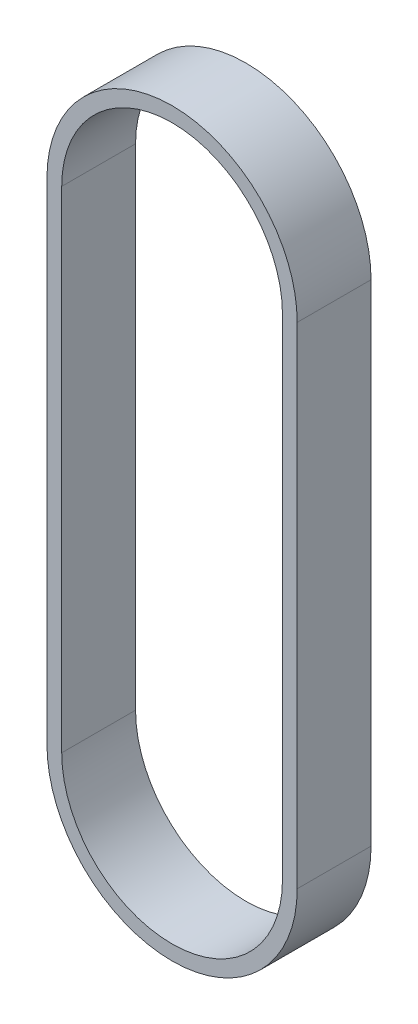
from build123d import *

# Parameters (mm, degrees)
EXTRUDE_THIN1_DEPTH = 10


with BuildPart() as part:
    # Sketch2 → Extrude-Thin1 (new body)
    with BuildSketch(Plane.XY):
        with BuildLine():
            Line((-30.341760221, -69.425568872), (-30.341760221, -3.000568872))
            ThreePointArc((-30.341760221, -3.000568872), (-13.396760221, 13.944431128), (3.548239779, -3.000568872))
            Line((3.548239779, -3.000568872), (3.548239779, -69.425568872))
            ThreePointArc((3.548239779, -69.425568872), (-13.396760221, -86.370568872), (-30.341760221, -69.425568872))
        make_face()
        with BuildLine():
            Line((-28.341760221, -69.425568872), (-28.341760221, -3.000568872))
            ThreePointArc((-28.341760221, -3.000568872), (-13.396760221, 11.944431128), (1.548239779, -3.000568872))
            Line((1.548239779, -3.000568872), (1.548239779, -69.425568872))
            ThreePointArc((1.548239779, -69.425568872), (-13.396760221, -84.370568872), (-28.341760221, -69.425568872))
        make_face(mode=Mode.SUBTRACT)
    extrude(amount=EXTRUDE_THIN1_DEPTH)


solid = part.part
